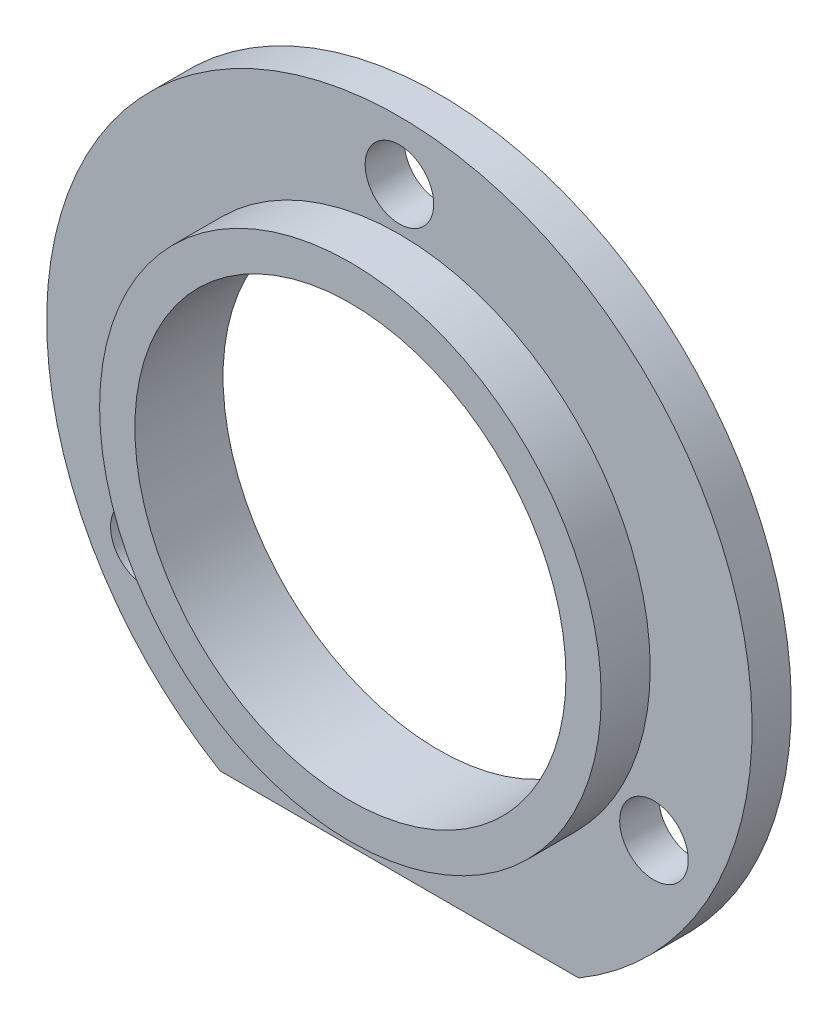
SolidWorks part; units mm, degrees
ref_plane "前视基准面" through (0, 0, 0) normal (0, 0, 1) x (1, 0, 0)
ref_plane "上视基准面" through (0, 0, 0) normal (0, 1, 0) x (1, 0, 0)
ref_plane "右视基准面" through (0, 0, 0) normal (1, 0, 0) x (0, 0, -1)
sketch "草图1" plane through (0, 0, 0) normal (0, 0, 1) x (1, 0, 0)
  line L0 (-82.3727, 0) -> (80.913, 0) construction
  line L1 (0, 76.0186) -> (0, -85.8157) construction
  circle A0 centre (0, 0) radius 11
  circle A1 centre (0, 0) radius 18
  dimension "D1" = 22
  dimension "D2" = 36
extrude "凸台-拉伸1" add sketch "草图1" along normal blind 4.5
sketch "草图2" plane through (0, 0, 4.5) normal (0, 0, 1) x (1, 0, 0)
  circle A0 centre (0, 0) radius 12.8
  dimension "D1" = 25.6
extrude "切除-拉伸1" cut sketch "草图2" against normal blind 2.5 flip side to cut
sketch "草图3" plane through (0, 0, 2) normal (0, 0, 1) x (1, 0, 0)
  line L0 (-24.7879, 0) -> (20.9968, 0) construction
  line L1 (-24.7879, -15.5) -> (20.9968, -15.5)
  line L2 (-24.7879, -15.5) -> (-24.7879, -20.8728)
  line L3 (-24.7879, -20.8728) -> (20.9968, -20.8728)
  line L4 (20.9968, -20.8728) -> (20.9968, -15.5)
  dimension "D1" = 15.5
extrude "切除-拉伸2" cut sketch "草图3" against normal through all
sketch "草图4" plane through (0, 0, 0) normal (0, 0, -1) x (-1, 0, 0)
  line L0 (-26.8438, 0) -> (22.6183, 0) construction
  line L1 (0, 22.3402) -> (0, -21.1216) construction
  line L2 (0, 0) -> (17.0843, -9.8636) construction
  line L3 (0, 0) -> (-19.689, -11.3674) construction
  circle A0 centre (0, 0) radius 15 construction
  circle A1 centre (0, 15) radius 1.75
  circle A2 centre (-12.9904, -7.5) radius 1.75
  circle A3 centre (12.9904, -7.5) radius 1.75
  dimension "D1" = 30
  dimension "D4" = 3.5
  dimension "D5" = 3.5
  dimension "D6" = 3.5
  dimension "D2" = 120
  dimension "D3" = 120
extrude "切除-拉伸3" cut sketch "草图4" against normal through all
